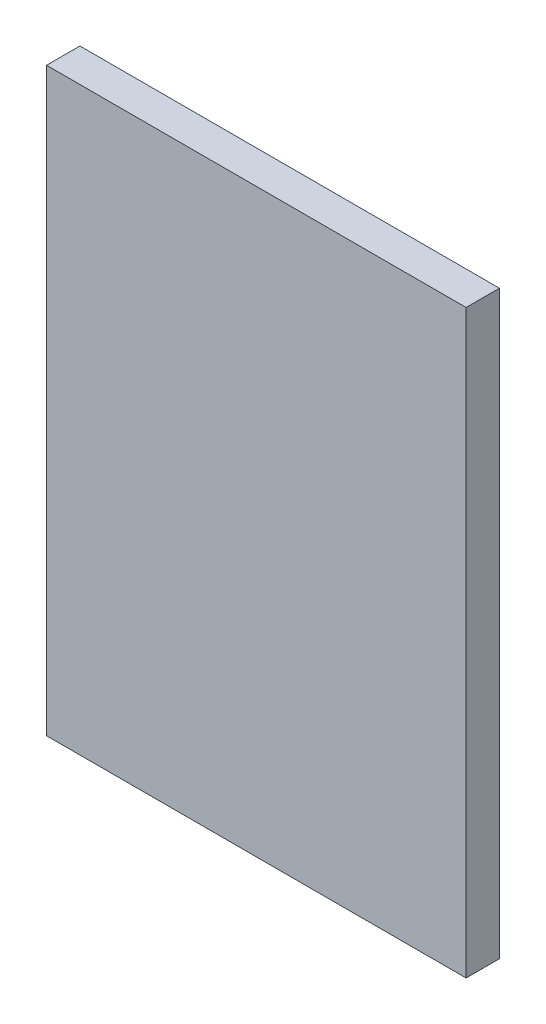
from build123d import *

# Parameters (mm, degrees)
SKETCH_1_W      = 151
SKETCH_1_H      = 209
EXTRUDE_1_DEPTH = 12


with BuildPart() as part:
    # 草图1 → 凸台-拉伸1 (new body)
    with BuildSketch(Plane.XY):
        Rectangle(SKETCH_1_W, SKETCH_1_H)
    extrude(amount=EXTRUDE_1_DEPTH)


solid = part.part
